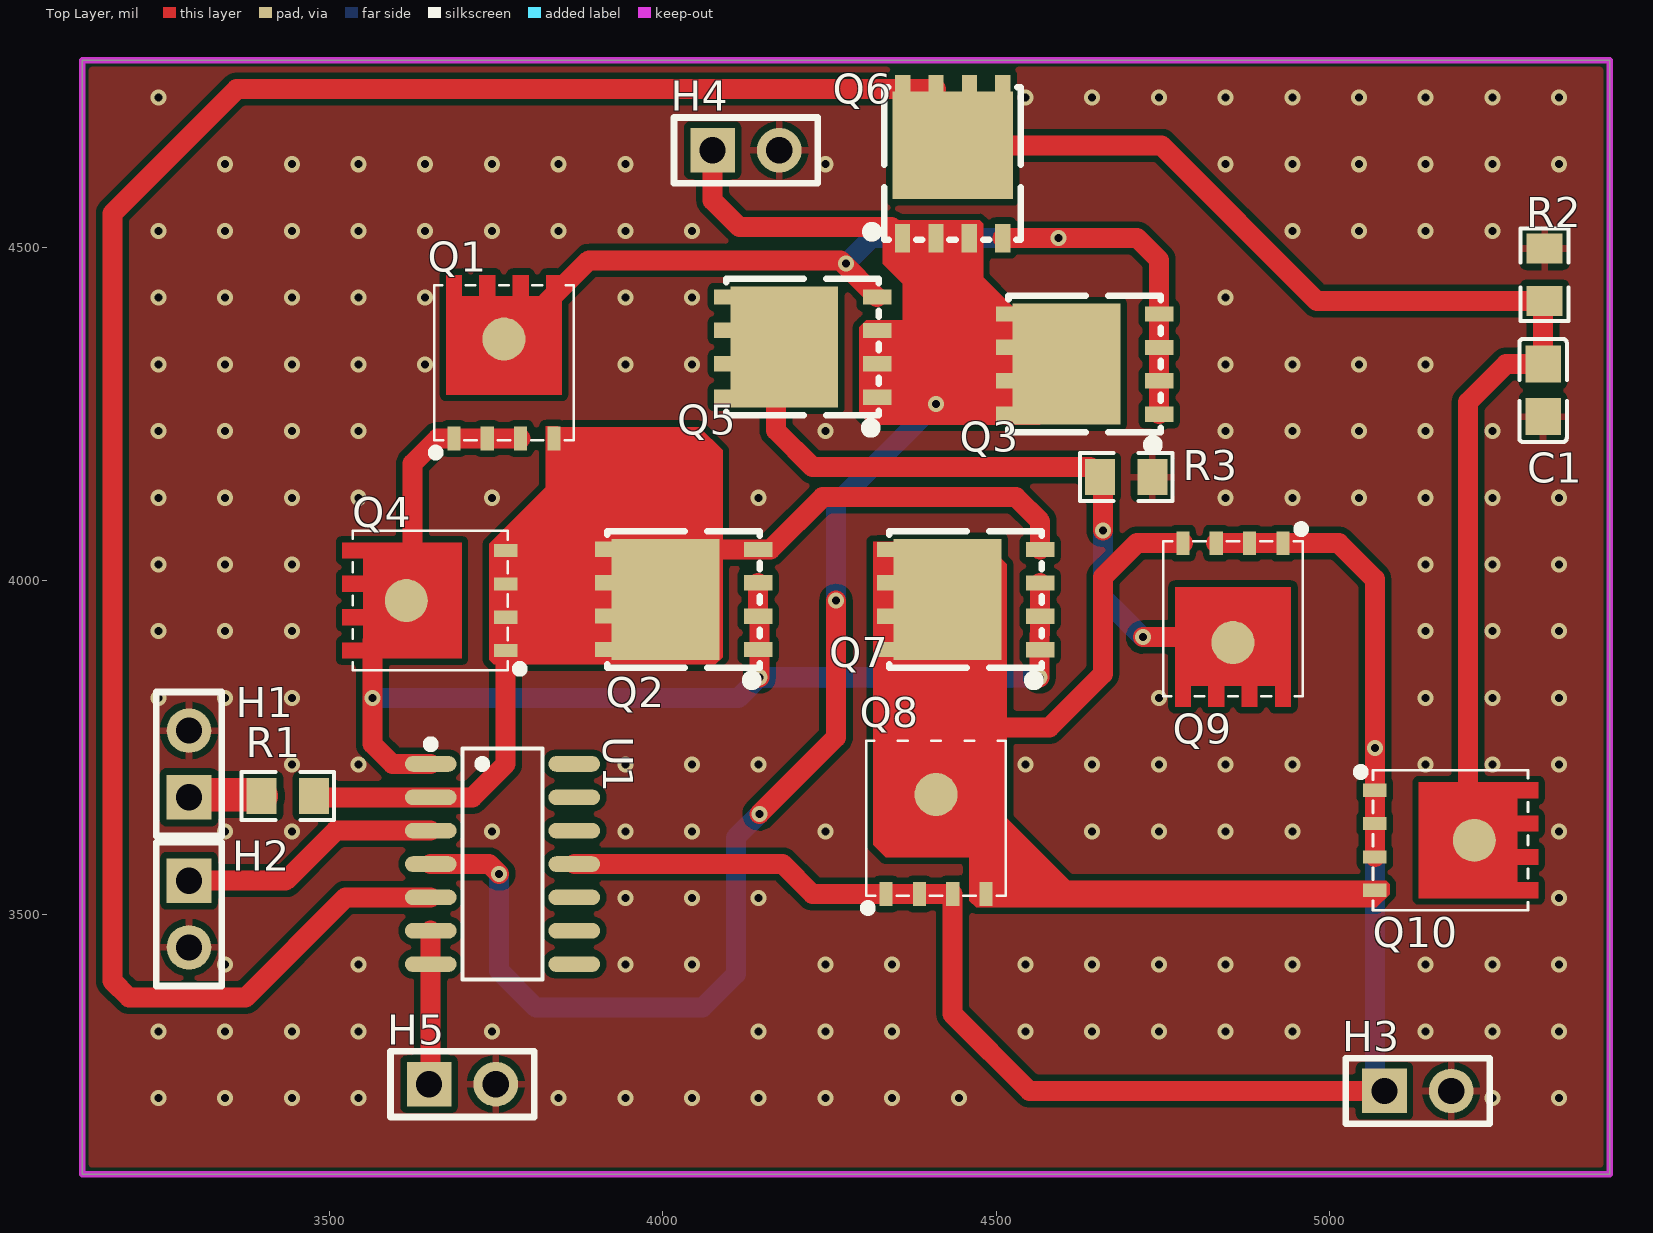
[diagram p0: Top Layer view]
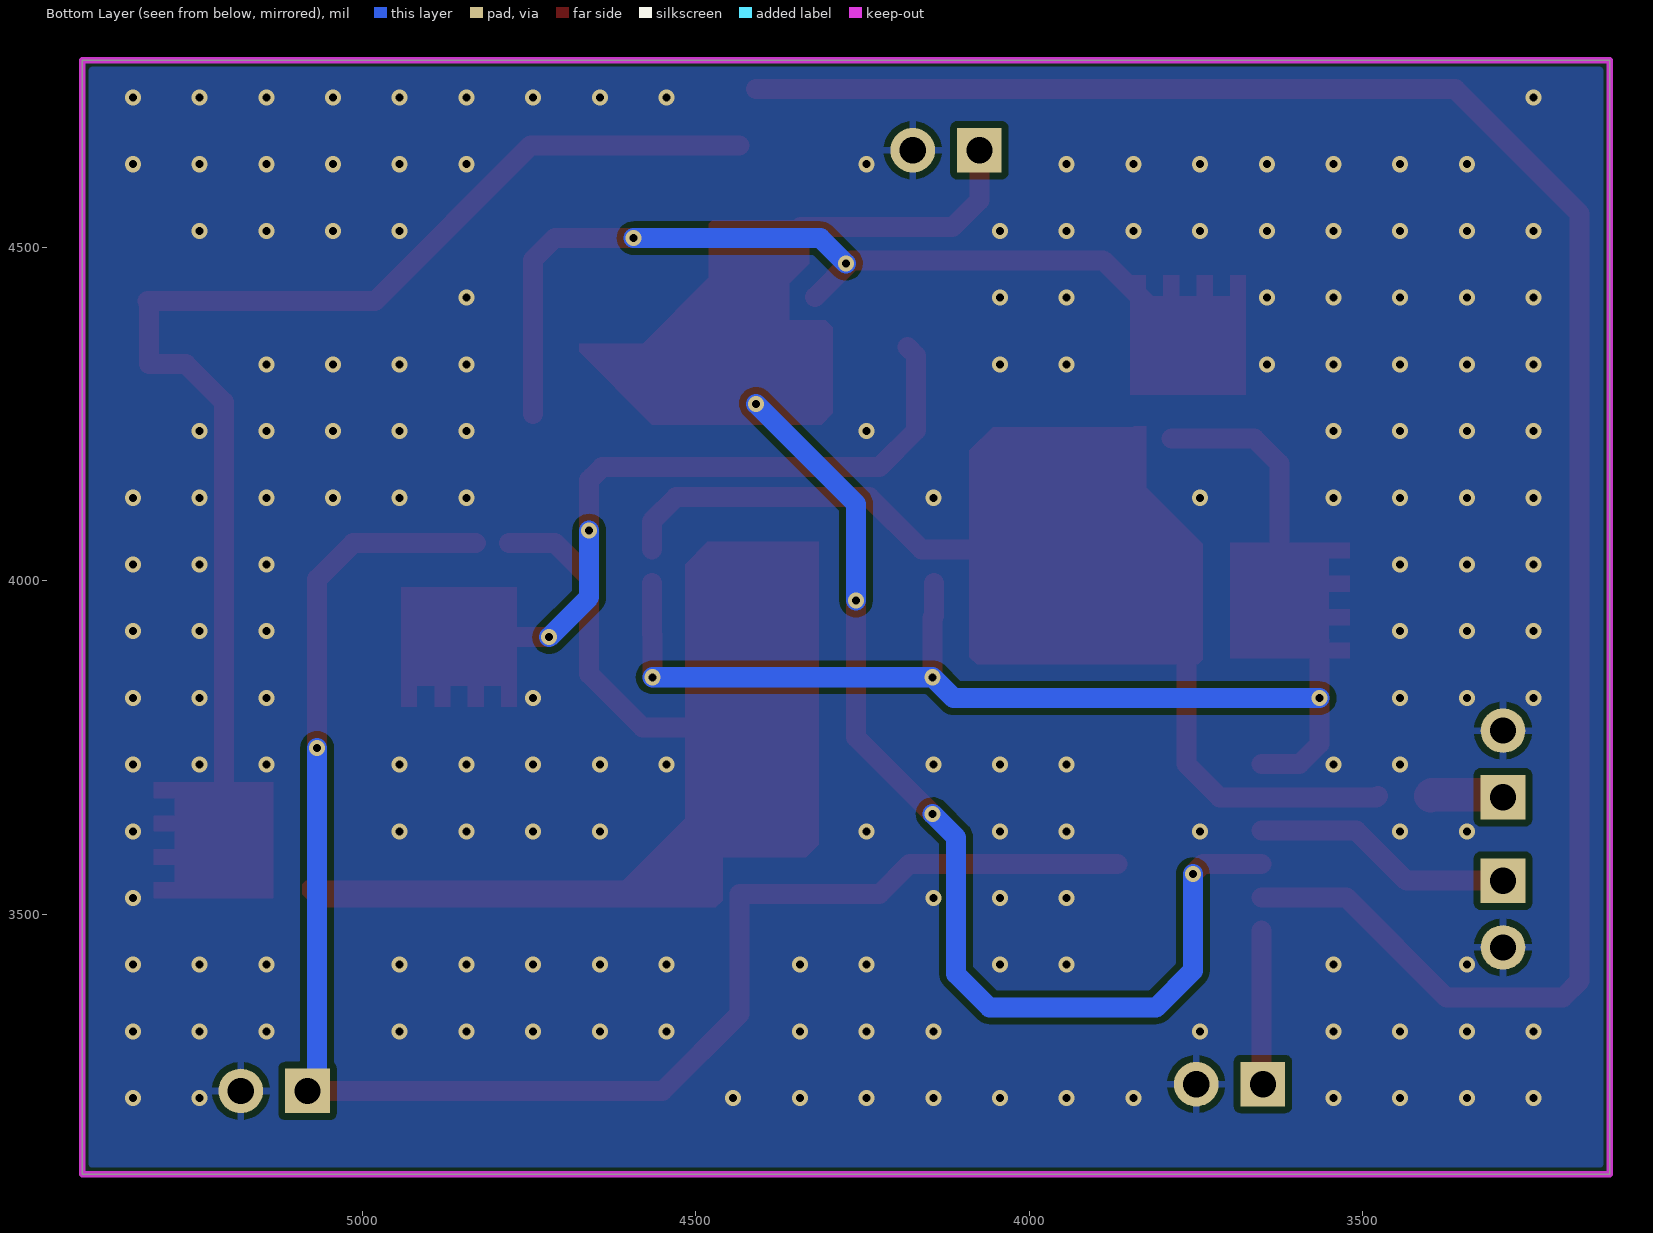
[diagram p1: Bottom Layer view, seen from below]
# Altium PCB MISC51994.pcbdoc
Units mil, origin at the board's own origin, x right, y up, seen from the top; angles counter-clockwise.
Board outline 2290 x 1670 mil, 2 copper layers (Top Layer, Bottom Layer), stack 62.206 mil thick; 20 components, 12 nets, 102 pads, 180 vias.

## Layer stack, top to bottom
Top Solder Mask Layer: solder mask 0.394, Dk 3.3
Top Layer: signal copper 1.379
Dielectric1: surface 59.449, FR4, Dk 4.5
Bottom Layer: signal copper 1.378
Bottom Solder Mask Layer: solder mask 0.394, Dk 3.3

## Board outline
3130,4780 3130,3110 5420,3110 5420,4780

## Design rules (kind name [scope] priority, off if disabled: settings)
BoardOutlineClearance copperThickness2oz_1 [All] p2 off: genericclearance=7.99 ignorepadtopadclearanceinfootprint=FALSE except(0: Arc-SplitContinuation Track-SplitContinuation SMDPad-SplitContinuation THPad-SplitContinuation Via-SplitContinuation Fill-SplitContinuation Region-SplitContinuation Poly-SplitContinuation Text-SplitContinuation Hole-SplitContinuation; 5.98: Arc-CutoutEdge SMDPad-CutoutEdge THPad-CutoutEdge Via-CutoutEdge Fill-CutoutEdge Region-CutoutEdge Text-CutoutEdge; 6.93: Hole-OutlineEdge Hole-CutoutEdge; 10: Poly-OutlineEdge Poly-CutoutEdge; 11.81: Arc-OutlineEdge Track-OutlineEdge SMDPad-OutlineEdge THPad-OutlineEdge Via-OutlineEdge Fill-OutlineEdge Region-OutlineEdge Text-OutlineEdge Track-CutoutEdge)
BoardOutlineClearance copperThickness1oz_1 [All] p4: genericclearance=4.02 ignorepadtopadclearanceinfootprint=FALSE except(0: Arc-SplitContinuation Track-SplitContinuation SMDPad-SplitContinuation THPad-SplitContinuation Via-SplitContinuation Fill-SplitContinuation Region-SplitContinuation Poly-SplitContinuation Text-SplitContinuation Hole-SplitContinuation; 6: SMDPad-CutoutEdge THPad-CutoutEdge Via-CutoutEdge Fill-CutoutEdge Region-CutoutEdge Text-CutoutEdge; 6.93: Hole-OutlineEdge Hole-CutoutEdge; 10: Poly-OutlineEdge Poly-CutoutEdge; 11.8: Arc-OutlineEdge Track-OutlineEdge SMDPad-OutlineEdge THPad-OutlineEdge Via-OutlineEdge Fill-OutlineEdge Region-OutlineEdge Text-OutlineEdge; 11.81: Arc-CutoutEdge Track-CutoutEdge)
Clearance copperThickness2oz [All] p1 off: gap=7.99 ignorepadtopadclearanceinfootprint=FALSE except(5.98: SMDPad-Track SMDPad-SMDPad THPad-Track SMDPad-THPad THPad-THPad Track-Via SMDPad-Via THPad-Via Via-Via Fill-Track Region-Track Fill-SMDPad Region-SMDPad Fill-THPad Region-THPad Fill-Via Region-Via Fill-Fill Fill-Region Region-Region Arc-Track Arc-SMDPad Arc-THPad Arc-Via Fill-Arc Region-Arc Arc-Arc Text-Track SMDPad-Text Text-THPad Text-Via Fill-Text Region-Text Arc-Text Text-Text; 6.93: Hole-Track Hole-SMDPad Hole-THPad Hole-Via Fill-Hole Region-Hole Hole-Arc Hole-Text; 10: Poly-Track Poly-SMDPad Poly-THPad Poly-Via Poly-Fill Poly-Region Poly-Poly Poly-Arc Poly-Text Poly-Hole)
Clearance copperThickness1oz [All] p3: gap=4.02 ignorepadtopadclearanceinfootprint=FALSE except(5.98: SMDPad-Track SMDPad-SMDPad THPad-Track SMDPad-THPad THPad-THPad Track-Via SMDPad-Via THPad-Via Via-Via Fill-Track Region-Track Fill-SMDPad Region-SMDPad Fill-THPad Region-THPad Fill-Via Region-Via Fill-Fill Fill-Region Region-Region; 6: Arc-Track Arc-SMDPad Arc-THPad Arc-Via Fill-Arc Region-Arc Arc-Arc Text-Track SMDPad-Text Text-THPad Text-Via Fill-Text Region-Text Arc-Text Text-Text; 6.93: Hole-Track Hole-SMDPad Hole-THPad Hole-Via Fill-Hole Region-Hole Hole-Arc Hole-Text; 10: Poly-Track Poly-SMDPad Poly-THPad Poly-Via Poly-Fill Poly-Region Poly-Poly Poly-Arc Poly-Text Poly-Hole)
DiffPairsRouting differentialPair [All] p1: maxlimit=6 minlimit=6 mostfreqgap=6 toplayer_minwidth=5 toplayer_prefwidth=10 toplayer_maxwidth=100 toplayer_mingap=6 toplayer_prefgap=6 toplayer_maxgap=6 bottomlayer_minwidth=5 bottomlayer_prefwidth=10 bottomlayer_maxwidth=100 bottomlayer_mingap=6 bottomlayer_prefgap=6 bottomlayer_maxgap=6 maxuncoupledlength=10
HoleToHoleClearance otherClearance [All] p1: gap=11.81 allowstackedmicrovias=TRUE
Length netLength [All] p1: minlimit=0 maxlimit=0
MatchedLengths netLengthTolerance [All] p1: tolerance=1000
PasteMaskExpansion pasteMaskExpansion [All] p1: expansion=0
PlaneConnect innerPlane [All] p1: planeconnectstyle=Relief reliefexpansion=20 reliefentries=4 reliefconductorwidth=10 reliefairgap=10
PolygonConnect copperRegion [(InNet('GND'))] p1: connectstyle=Relief reliefconductorwidth=10 reliefentries=4 polygonreliefangle="90 Angle" airgapwidth=10 via.connectstyle=Relief via.reliefconductorwidth=10 via.reliefentries=4 via.polygonreliefangle="90 Angle" via.airgapwidth=10
RoutingVias viaSize [All] p1: holewidth=12.01 width=24.02 viastyle="Through Hole" minholewidth=11.81 minwidth=19.68 maxholewidth=248.03 maxwidth=393.7
SolderMaskExpansion solderMaskExpansion [IsVia] p1: expansion=-1000 istentingtop=TRUE
SolderMaskExpansion solderMaskExpansion [All] p2: expansion=2 istentingtop=FALSE
Width copperThickness2oz_2 [All] p1 off: maxlimit=100 minlimit=8 preferedwidth=10
Width copperThickness1oz_2 [All] p2: maxlimit=100 minlimit=5 preferedwidth=10

## Components (designator, comment, footprint, x,y, rotation, side; value= is the part's Value field where it differs from the comment)
C1 "3.3nF" C0805 5320,4285 r90 top
H1 "" HDR-TH_2P-P2.54-V-F 3290,3725 r90 top
H2 "" HDR-TH_2P-P2.54-V-F 3290,3500 r270 top
H3 "" HDR-TH_2P-P2.54-V-F 5132.21,3234.84 r0 top
H4 "" HDR-TH_2P-P2.54-V-F 4125,4645 r0 top
H5 "" HDR-TH_2P-P2.54-V-F 3700,3245 r0 top
Q1 "SI7336ADP-T1-E3-MS" TDSON-8_L5.9-W5.2-P1.27-BL-1 3762.21,4282.8 r0 top
Q2 "AON6407" PDFN-8_L4.9-W5.8-P1.27-LS6.1-BL 4031.69,3971.68 r90 top
Q3 "AON6407" PDFN-8_L4.9-W5.8-P1.27-LS6.1-BL 4632.95,4324.52 r90 top
Q4 "SI7336ADP-T1-E3-MS" TDSON-8_L5.9-W5.2-P1.27-BL-1 3695,3970 r90 top
Q5 "AON6407" PDFN-8_L4.9-W5.8-P1.27-LS6.1-BL 4210,4350 r90 top
Q6 "AON6407" PDFN-8_L4.9-W5.8-P1.27-LS6.1-BL 4435,4625 r0 top
Q7 "AON6407" PDFN-8_L4.9-W5.8-P1.27-LS6.1-BL 4454.48,3971.47 r90 top
Q8 "SI7336ADP-T1-E3-MS" TDSON-8_L5.9-W5.2-P1.27-BL-1 4410,3600 r0 top
Q9 "SI7336ADP-T1-E3-MS" TDSON-8_L5.9-W5.2-P1.27-BL-1 4855.07,3986.23 r180 top
Q10 "SI7336ADP-T1-E3-MS" TDSON-8_L5.9-W5.2-P1.27-BL-1 5137.79,3610.59 r270 top
R1 "47K" R0805 3438.2,3677 r0 top
R2 "1e9" R0805 5322.42,4458.41 r270 top
R3 "1e6" R0805 4695,4155 r180 top
U1 "TL084" SOP-14_L8.6-W3.9-P1.27-LS6.0-BL 3760,3575 r270 top

## Footprints (in the part's own frame and the unit in brackets; to place one, negate y for a bottom-side part, rotate by r counter-clockwise, add the part's x,y. Pads: shape width x height; smd on the part's side, far side on the other; paste and mask are expansions set on the pad)
C0805 [mm]
  rect 1.41x1.35 smd paste-100 mask+0.051: 1(-1,0) 2(1,0)
  silkscreen extent -1.96,-0.9 1.96,0.9
HDR-TH_2P-P2.54-V-F [mm]
  rect 1.7x1.7 hole 1: 1(-1.27,0)
  round 1.7 hole 1: 2(1.27,0)
  silkscreen extent -2.74,-1.25 2.74,1.25
PDFN-8_L4.9-W5.8-P1.27-LS6.1-BL [mm]
  rect 0.58x1.079 smd paste-100 mask+0.05: 1(-1.907,-2.835) 2(-0.637,-2.835) 3(0.633,-2.835) 4(1.903,-2.835)
  rect 0.58x1.08 smd paste-100 mask+0.05: 5(1.907,2.835) 6(0.638,2.835) 7(-0.632,2.835) 8(-1.902,2.835)
  rect 4.6x4.1 smd paste-100 mask+0.05: 9(-0.002,0.695)
  silkscreen extent -3.2,-2.89 2.6,2.9
R0805 [mm]
  rect 1.133x1.377 smd paste-100 mask+0.051: 1(-1,0) 2(1,0)
  silkscreen extent -1.76,-0.92 1.76,0.92
SOP-14_L8.6-W3.9-P1.27-LS6.0-BL [mm]
  oval 0.595x1.968 smd: 1(-3.81,-2.734) 2(-2.54,-2.734) 3(-1.27,-2.734) 4(0,-2.734) 5(1.27,-2.734) 6(2.54,-2.734) 7(3.81,-2.734) 8(3.81,2.734) 9(2.54,2.734) 10(1.27,2.734) 11(0,2.734) 12(-1.27,2.734) 13(-2.54,2.734) 14(-3.81,2.734)
  silkscreen extent -4.71,-2.88 4.4,1.52
TDSON-8_L5.9-W5.2-P1.27-BL-1 [mm]
  rect 0.5x0.9 smd paste-100 mask+0.05: 1(-1.905,-1.775) 2(-0.635,-1.775) 3(0.635,-1.775) 4(1.905,-1.775)
  round 1.638 smd: 5(0,2.012)
  Top Layer region: -2.205,-0.1 2.205,-0.1 2.205,4.45 1.605,4.45 1.605,3.65 0.935,3.65 0.935,4.45 0.335,4.45 0.335,3.65 -0.335,3.65 -0.335,4.45 -0.935,4.45 -0.935,3.65 -1.605,3.65 -1.605,4.45 -2.205,4.45
  silkscreen extent -2.75,-2.46 2.66,4.06

## Via types
v1: diameter 24.02, hole 12, Top Layer to Bottom Layer, 180 vias

## Nets (pads, with @x,y where several pads share a name; then routed paths per layer and width w, separated by ;. In a path a pad name is that pad's centre, name@x,y a point inside that pad or via, vN(x,y) a via of type N, cw(c..) or ccw(c..) an arc to the next point about the centre after c; other vN are vias at no path point)
$1N2: H1.1 R1.1 | length 116.8
  Top Layer w50: H1.1@3282.87,3679 3396.84,3679 R1.1
$1N3: Q1.4 Q2.4 Q2.5 Q2.6 Q2.7 Q2.8 Q2.9 Q4.1 Q4.2 Q4.3 Q4.4 Q7.4 R1.2 U1.2 | length 1161.6
  Top Layer w30: R1.2 3479.57,3675 U1.2 3715,3675 3764.88,3724.88 Q4.1 ; Q2.9 4079.33,4046.58 Q2.4 4161.58,4046.58 4240,4125 4529.88,4125 4566.08,4088.8 Q7.4
$1N4: H2.1 U1.3 | length 393.4
  Top Layer w30: H2.1 3435,3550 3510,3625 U1.3
$1N6: H3.1 Q8.1 Q8.2 Q8.3 Q9.1 Q9.2 Q9.3 Q10.1 Q10.2 Q10.3 U1.11 | length 2657.9
  Top Layer w30: U1.11 4180,3575 4224.88,3530.12 Q8.1 Q8.2 Q8.3 4435,3350 4550.16,3234.84 H3.1 ; Q9.3 Q9.2 Q9.1 5013.89,4056.11 5067.91,4002.09 v1(5067.91,3749.13) Q10.1 Q10.2 Q10.3
  Bottom Layer w30: v1(5067.91,3749.13) 5067.91,3249.15 H3.1
$1N8: Q1.1 Q1.2 Q1.3 Q2.1 Q2.2 Q2.3 Q4.5 Q7.1 Q7.2 Q7.3 U1.1 | length 2019.7
  Top Layer w30: U1.1 3595,3725 3565,3755 v1(3565,3823.68) 3565,3909.88 3625.12,3970 3625.12,4175.12 3662.92,4212.92 Q1.1 Q1.2 Q1.3 ; Q2.3 Q2.2 4145,3944.87 v1(4145,3855) ; v1(4565,3855) 4565,3919.02 4566.08,3920.1 Q7.2 Q7.3
  Bottom Layer w30: v1(3565,3823.68) 4113.68,3823.68 v1(4145,3855) v1(4565,3855)
$1N18: Q5.5 Q5.6 Q5.7 Q5.8 Q5.9 Q9.5 R3.2 | length 1047.1
  Top Layer w30: Q5.9 4170,4337.26 4170,4225 4225,4170 4640.63,4170 R3.2 4660,4150.63 v1(4660,4075) ; v1(4720,3915) 4853.73,3915 Q9.5@4855.07,3916.35
  Bottom Layer w30: v1(4660,4075) 4660,3975 v1(4720,3915)
$1N20: C1.2 Q6.5 Q6.6 Q6.7 Q6.8 Q6.9 Q10.5 R2.2 U1.5 | length 4885
  Top Layer w30: U1.5 3525,3525 3375,3375 3200,3375 3175,3400 3175,4550 3361.6,4736.6 Q6.8 Q6.7 ; Q6.9 4747.64,4652.36 4980.96,4419.04 R2.2 5320,4416.62 C1.2 5264.37,4324.37 5207.67,4267.67 Q10.5@5207.67,3610.59
$1N24: Q1.5 Q3.1 Q3.2 Q3.3 Q3.4 Q5.4 Q6.4 | length 1448.5
  Top Layer w30: Q1.5@3762.21,4352.68 3889.54,4480 4266.5,4480 Q5.4 ; Q6.4 v1(4593.33,4513.4) 4711.6,4513.4 4744.55,4480.45 Q3.4 Q3.3 Q3.2 Q3.1
  Bottom Layer w30: v1(4275,4475) 4313.4,4513.4 v1(4593.33,4513.4)
$1N33: H4.1 Q3.5 Q3.6 Q3.7 Q3.8 Q3.9 Q5.1 Q5.2 Q5.3 Q6.1 Q6.2 Q6.3 U1.4 | length 2014.9
  Top Layer w30: U1.4 3740,3575 v1(3755,3560) ; H4.1 4075,4570 4115,4530 4343.3,4530 Q6.1 ; v1(4145,3650) 4260,3765 v1(4260,3970)
  Bottom Layer w30: v1(3755,3560) 3755,3415 3810,3360 4060,3360 4110,3410 4110,3615 v1(4145,3650) ; v1(4260,3970) 4260,4115 v1(4410,4265)
$1N39: Q7.5 Q7.6 Q7.7 Q7.8 Q7.9 Q8.4 Q8.5 Q9.4 Q10.4 | length 509.4
  Top Layer w30: 4470,3780 4580,3780 4660,3860 4660,4005 4711.11,4056.11 Q9.4
GND: C1.1 H1.2 H2.2 H3.2 H4.2 H5.2 R2.1 R3.1
  other v1: 3244.1,3224.1 3344.1,3224.1 3444.1,3224.1 3544.1,3224.1 3844.1,3224.1 3944.1,3224.1 4044.1,3224.1 4144.1,3224.1 4244.1,3224.1 4344.1,3224.1 4444.1,3224.1 5244.1,3224.1 5344.1,3224.1 3244.1,3324.1 3344.1,3324.1 3444.1,3324.1 3544.1,3324.1 3744.1,3324.1 4144.1,3324.1 4244.1,3324.1 4344.1,3324.1 4544.1,3324.1 4644.1,3324.1 4744.1,3324.1 4844.1,3324.1 4944.1,3324.1 5144.1,3324.1 5244.1,3324.1 5344.1,3324.1 3344.1,3424.1 3544.1,3424.1 3944.1,3424.1 4044.1,3424.1 4244.1,3424.1 4344.1,3424.1 4544.1,3424.1 4644.1,3424.1 4744.1,3424.1 4844.1,3424.1 4944.1,3424.1 5144.1,3424.1 5244.1,3424.1 5344.1,3424.1 3944.1,3524.1 4044.1,3524.1 4144.1,3524.1 5344.1,3524.1 3344.1,3624.1 3444.1,3624.1 3744.1,3624.1 3944.1,3624.1 4044.1,3624.1 4244.1,3624.1 4644.1,3624.1 4744.1,3624.1 4844.1,3624.1 4944.1,3624.1 5344.1,3624.1 3444.1,3724.1 3544.1,3724.1 3944.1,3724.1 4044.1,3724.1 4144.1,3724.1 4544.1,3724.1 4644.1,3724.1 4744.1,3724.1 4844.1,3724.1 4944.1,3724.1 5144.1,3724.1 5244.1,3724.1 5344.1,3724.1 3244.1,3824.1 3344.1,3824.1 3444.1,3824.1 4744.1,3824.1 5144.1,3824.1 5244.1,3824.1 5344.1,3824.1 3244.1,3924.1 3344.1,3924.1 3444.1,3924.1 5144.1,3924.1 5244.1,3924.1 5344.1,3924.1 3244.1,4024.1 3344.1,4024.1 3444.1,4024.1 5144.1,4024.1 5244.1,4024.1 5344.1,4024.1 3244.1,4124.1 3344.1,4124.1 3444.1,4124.1 3544.1,4124.1 3744.1,4124.1 4144.1,4124.1 4844.1,4124.1 4944.1,4124.1 5044.1,4124.1 5144.1,4124.1 5244.1,4124.1 5344.1,4124.1 3244.1,4224.1 3344.1,4224.1 3444.1,4224.1 3544.1,4224.1 4244.1,4224.1 4844.1,4224.1 4944.1,4224.1 5044.1,4224.1 5144.1,4224.1 5244.1,4224.1 3244.1,4324.1 3344.1,4324.1 3444.1,4324.1 3544.1,4324.1 3644.1,4324.1 3944.1,4324.1 4044.1,4324.1 4844.1,4324.1 4944.1,4324.1 5044.1,4324.1 5144.1,4324.1 3244.1,4424.1 3344.1,4424.1 3444.1,4424.1 3544.1,4424.1 3644.1,4424.1 3944.1,4424.1 4044.1,4424.1 4844.1,4424.1 3244.1,4524.1 3344.1,4524.1 3444.1,4524.1 3544.1,4524.1 3644.1,4524.1 3744.1,4524.1 3844.1,4524.1 3944.1,4524.1 4044.1,4524.1 4944.1,4524.1 5044.1,4524.1 5144.1,4524.1 5244.1,4524.1 3344.1,4624.1 3444.1,4624.1 3544.1,4624.1 3644.1,4624.1 3744.1,4624.1 3844.1,4624.1 3944.1,4624.1 4244.1,4624.1 4844.1,4624.1 4944.1,4624.1 5044.1,4624.1 5144.1,4624.1 5244.1,4624.1 5344.1,4624.1 3244.1,4724.1 4544.1,4724.1 4644.1,4724.1 4744.1,4724.1 4844.1,4724.1 4944.1,4724.1 5044.1,4724.1 5144.1,4724.1 5244.1,4724.1 5344.1,4724.1
VC: H5.1 U1.6 U1.7 | length 231
  Top Layer w30: H5.1 3652.37,3247.37 U1.7 U1.6
pads on no net: U1.8 U1.9 U1.10 U1.12 U1.13 U1.14

## Polygon pours and split planes (outlines as drawn)
GND on Top Layer (solid, remove dead copper, pour order 0): 3000,4870 3000,3000 5530,3000 5530,4870
GND on Bottom Layer (solid, remove dead copper, pour order 2): 3000,4885 3000,3000 5500,3000 5500,4885

## Keep-outs
Board Outline Layer:
  the board outline again, w10

## Other copper
Top Layer:
  region net $1N3: 3824.73,4231.03 3843.97,4231.03 3845,4230 4055,4230 4090,4195 4090,3885 4079.14,3874.14 3746.77,3874.14 3740,3880.91 3740,4055 3824.73,4139.73
  region net $1N33: 4340,4540 4475.38,4540 4480.54,4534.84 4480.54,4454.46 4580,4355 4675,4355 4675,4342.91 4565.98,4233.89 4311.72,4233.89 4294.71,4250.9 4294.71,4379.71 4305,4390 4360,4390 4360,4445 4330,4475 4330,4530
  region net $1N39: 4315.48,4057.97 4482.66,4057.97 4516.24,4024.39 4516.24,3643.76 4610,3550 5085,3550 5090,3545 5090,3530 5070,3510 4470,3510 4460,3520 4460,3585 4334.25,3585 4315.48,3603.77